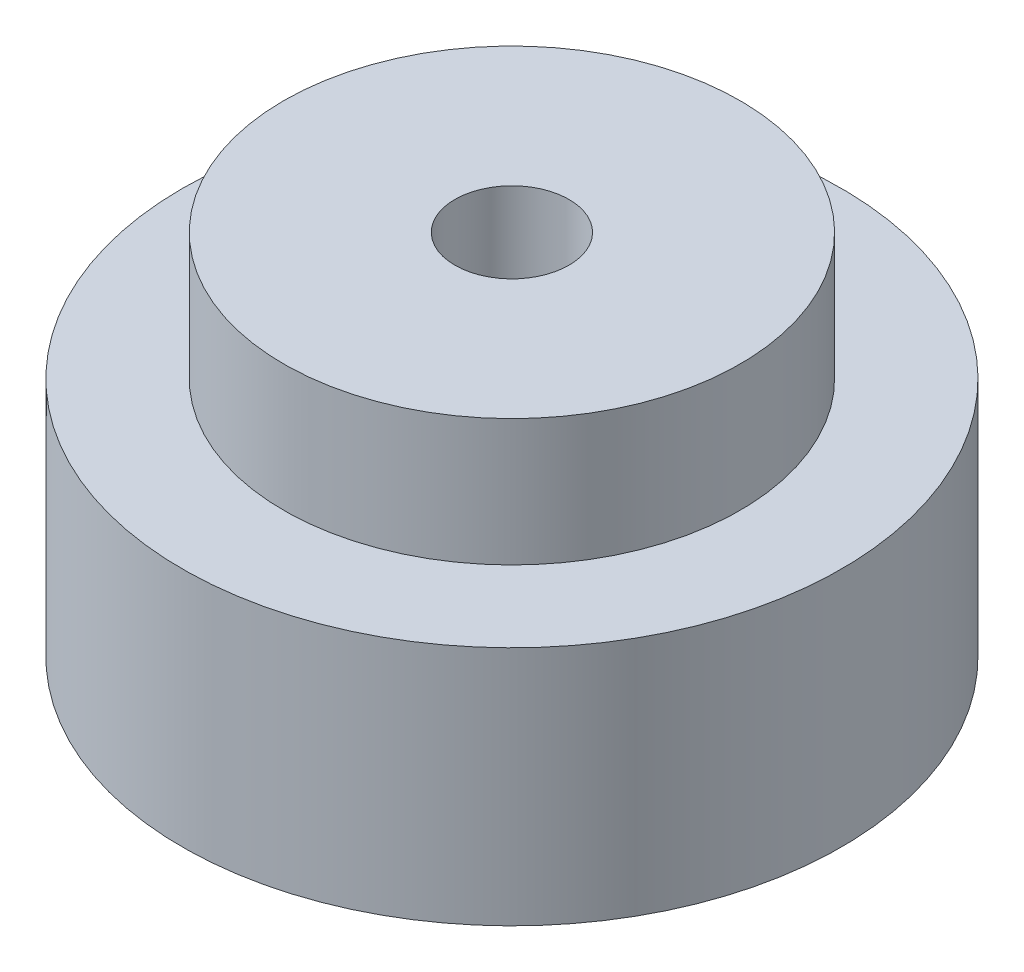
SolidWorks part; units mm, degrees
material "1.0503 (C45)"
ref_plane "前视基准面" through (0, 0, 0) normal (0, 0, 1) x (1, 0, 0)
ref_plane "上视基准面" through (0, 0, 0) normal (0, 1, 0) x (1, 0, 0)
ref_plane "右视基准面" through (0, 0, 0) normal (1, 0, 0) x (0, 0, -1)
sketch "草图1" plane through (0, 0, 0) normal (0, 0, 1) x (1, 0, 0)
  line L0 (20, 0) -> (26, 0)
  line L1 (0, 29.7122) -> (0, -13.6211) construction
  line L2 (26, 0) -> (26, 19)
  line L3 (26, 19) -> (18, 19)
  line L4 (18, 19) -> (18, 29)
  line L5 (18, 29) -> (0, 29)
  line L6 (0, 29) -> (0, 17)
  line L7 (-37.6561, 0) -> (41.7766, 0) construction
  line L8 (20, 11) -> (20, 0)
  line L9 (20, 11) -> (5, 17)
  line L10 (5, 17) -> (0, 17)
  dimension "D1" = 52
  dimension "D2" = 36
  dimension "D3" = 19
  dimension "D4" = 29
  dimension "D5" = 10
  dimension "D6" = 40
  dimension "D7" = 11
  dimension "D8" = 12
revolve "旋转1" add sketch "草图1" angle 360 about L1
hole_wizard "M10x1.0 螺纹孔1" positions "草图3" profile "草图2" tap size "M10x1.0" standard "GB" end condition up to next
sketch "草图3" plane through (0, 29, 0) normal (0, 1, 0) x (1, 0, 0)
  point P0 (0, 0)
sketch "草图2" plane through (0, 29, 0) normal (1, 0, 0) x (0, 0, 1)
  line L0 (0, 0) -> (0, 12)
  line L1 (0, 12) -> (4.5, 12)
  line L2 (4.5, 12) -> (4.5, 0)
  line L5 (4.5, 0) -> (0, 0)
  line L11 (0, -6.35) -> (0, 107.95) construction
  dimension "通孔螺纹孔钻头直径" = 9
  dimension "通孔螺纹孔钻头深度" = 12
cosmetic thread "孔螺蚊线1" parameters "D2"=10
sketch "草图4" plane through (0, 0, 0) normal (1, 0, 0) x (0, 0, -1)
  line L0 (0, 41.9025) -> (0, -9.7091) construction
  line L1 (-26, 0) -> (26, 0) construction
  line L2 (-26, 0) -> (26, 0) construction
  circle A0 centre (0, 9) radius 3
  dimension "D2" = 6
  dimension "D1" = 9
extrude "切除-拉伸1" cut sketch "草图4" against normal through all
